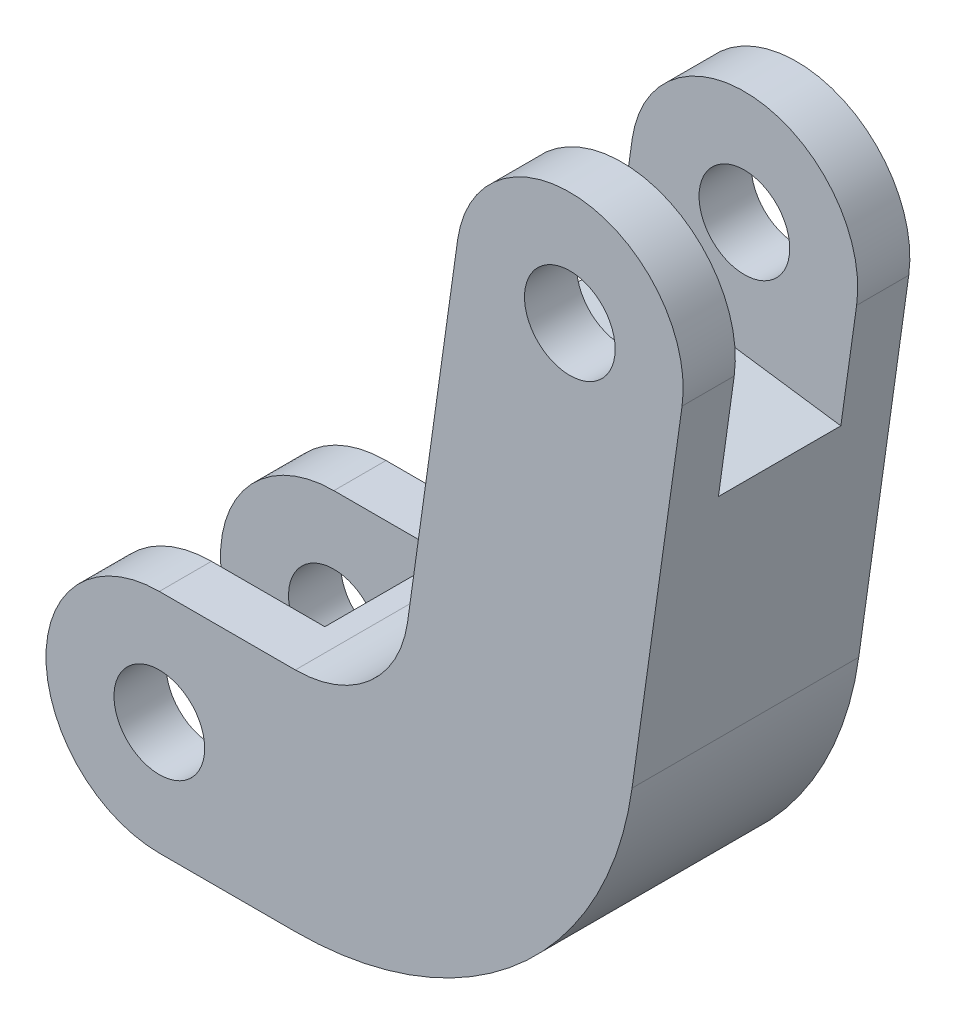
SolidWorks part; units mm, degrees
other "Annotation1"
sketch "草图8" plane through (40.3641, 54.3041, 5) normal (0.8399, 0.4737, 0.265) x (0.2751, 0.0494, -0.9602)
ref_plane "Front Plane" through (0, 0, 0) normal (0, 0, 1) x (1, 0, 0)
ref_plane "Top Plane" through (0, 0, 0) normal (0, 1, 0) x (1, 0, 0)
ref_plane "Right Plane" through (0, 0, 0) normal (1, 0, 0) x (0, 0, -1)
other "Configuration Table"
sketch "Sketch1" plane through (0, 0, 0) normal (0, 0, 1) x (1, 0, 0)
  line L0 (10.9513, 4.3041) -> (13.1573, 20)
  line L1 (0, 0) -> (6, 0)
  line L2 (0, 0) -> (0, 56.2449) construction
  line L3 (0, -10) -> (6, -10)
  line L4 (20.854, 2.9124) -> (23.0599, 18.6083)
  arc A0 (6, 0) -> (10.9513, 4.3041) centre (6, 5) ccw
  arc A1 (6, -10) -> (20.854, 2.9124) centre (6, 5) ccw
  arc A2 (13.1573, 20) -> (23.0599, 18.6083) centre (18.1086, 19.3041) cw
  arc A3 (0, 0) -> (0, -10) centre (0, -5) ccw
  dimension "D1" = 5
  dimension "D2" = 20
  dimension "D3" = 8
  dimension "D4" = 6
  dimension "D5" = 10
extrude "Boss-Extrude1" add sketch "Sketch1" along normal mid plane 10
sketch "Sketch2" plane through (0, 0, 0) normal (0, 0, 1) x (1, 0, 0)
  circle A1 centre (0, -5) radius 2
  dimension "D1" = 4
extrude "Cut-Extrude1" cut sketch "Sketch2" against normal through all both and the other way through all
ref_plane "Plane1" through (-5, 0, 0) normal (1, 0, 0) x (0, 0, -1)
sketch "Sketch3" plane through (-5, 0, 0) normal (1, 0, 0) x (0, 0, -1)
  line L0 (-5, 0) -> (5, 0) construction
  line L1 (2.7, 0) -> (-2.7, 0)
  line L2 (2.7, 0) -> (2.7, -10)
  line L3 (2.7, -10) -> (-2.7, -10)
  line L4 (-2.7, 0) -> (-2.7, -10)
  line L5 (-5, -10) -> (5, -10) construction
  line L6 (0, 0) -> (0, -10) construction
  dimension "D1" = 5.4
extrude "Cut-Extrude2" cut sketch "Sketch3" along normal blind 10
sketch "Sketch4" plane through (0, 0, 5) normal (0, 0, 1) x (1, 0, 0)
  circle A0 centre (18.1086, 19.3041) radius 2
  dimension "D1" = 4
extrude "Cut-Extrude3" cut sketch "Sketch4" against normal blind 31
sketch "Sketch7" plane through (20.0487, -2.8177, 0) normal (0.9903, -0.1392, 0) x (0, 0, -1)
  line L0 (5, 26.6365) -> (-5, 26.6365) construction
  line L1 (2.7, 26.6365) -> (-2.7, 26.6365)
  line L2 (2.7, 26.6365) -> (2.7, 16.6365)
  line L3 (2.7, 16.6365) -> (-2.7, 16.6365)
  line L4 (-2.7, 26.6365) -> (-2.7, 16.6365)
  line L5 (0, 26.6365) -> (0, 16.6365) construction
  dimension "D1" = 10
  dimension "D2" = 5.4
extrude "Cut-Extrude5" cut sketch "Sketch7" against normal blind 13
